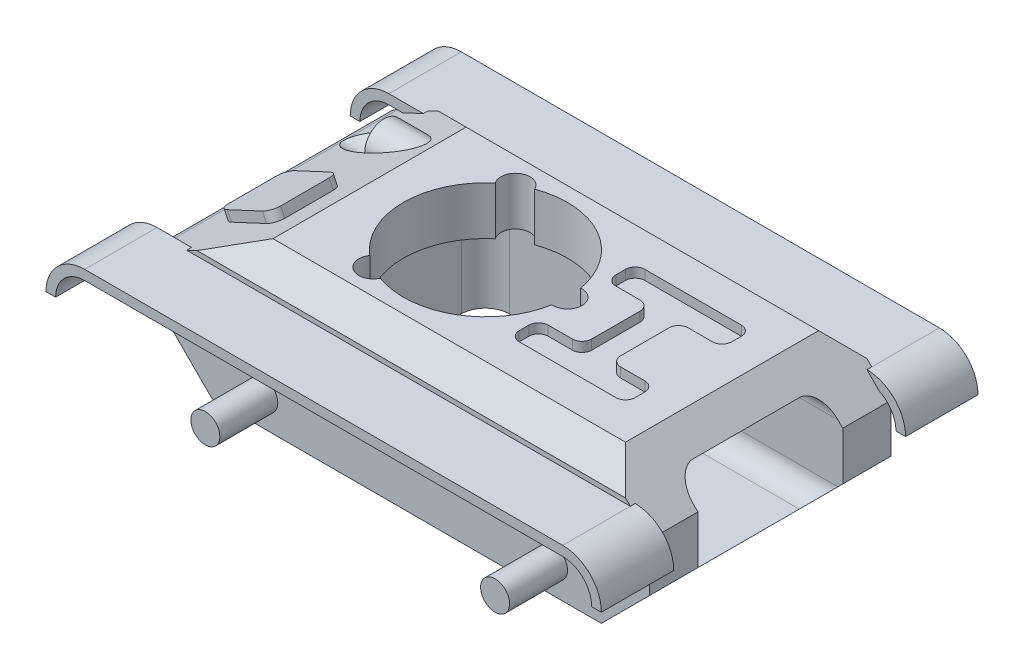
SolidWorks part; units mm, degrees
ref_plane "Front Plane" through (0, 0, 0) normal (0, 0, 1) x (1, 0, 0)
ref_plane "Top Plane" through (0, 0, 0) normal (0, 1, 0) x (1, 0, 0)
ref_plane "Right Plane" through (0, 0, 0) normal (1, 0, 0) x (0, 0, -1)
sketch "Sketch1" plane through (0, 0, 0) normal (0, 0, 1) x (1, 0, 0)
  line L0 (0, 0) -> (-80.6266, 0)
  line L1 (-80.6266, 0) -> (-93.6115, 12.9849)
  line L2 (-92.1891, 21.052) -> (-73, 30)
  line L3 (-73, 30) -> (0, 30)
  line L4 (0, 30) -> (10, 20)
  line L5 (10, 20) -> (10, 10)
  line L6 (10, 10) -> (0, 0)
  arc A0 (-92.1891, 21.052) -> (-93.6115, 12.9849) centre (-90.076, 16.5205) ccw
  point P12 (-95, 17.3887)
  dimension "D2" = 5
  dimension "D1" = 70
  dimension "D3" = 30
  dimension "D4" = 45
  dimension "D5" = 45
  dimension "D6" = 10
  dimension "D7" = 45
  dimension "D8" = 10
  dimension "D9" = 105
  dimension "D10" = 22
extrude "Boss-Extrude1" add sketch "Sketch1" along normal mid plane 50
chamfer "Chamfer1" distance 5 angle 45 2 edges at (-36.5, 30, 25) (-36.5, 30, -25)
sketch "Sketch2" plane through (0, 30, 0) normal (0, 1, 0) x (1, 0, 0)
  line L4 (-14, -7) -> (-9, -7)
  line L5 (-7, -9) -> (-7, -11)
  line L6 (-9, -13) -> (-29, -13)
  line L7 (-31, -11) -> (-31, -9)
  line L8 (-29, -7) -> (-24, -7)
  line L9 (-22, -5) -> (-22, 5)
  line L12 (10, -25) -> (10, 25) construction
  line L13 (-49, 0) -> (21.9444, 0) construction
  line L14 (-16, -5) -> (-16, 5)
  line L15 (-29, 7) -> (-24, 7)
  line L16 (-31, 11) -> (-31, 9)
  line L17 (-9, 13) -> (-29, 13)
  line L18 (-7, 9) -> (-7, 11)
  line L19 (-14, 7) -> (-9, 7)
  arc A0 (-59.9556, 12.999) -> (-59.9556, -12.999) centre (-49, 0) ccw
  arc A3 (-7, -11) -> (-9, -13) centre (-9, -11) cw
  arc A4 (-9, -7) -> (-7, -9) centre (-9, -9) cw
  arc A5 (-29, -13) -> (-31, -11) centre (-29, -11) cw
  arc A6 (-31, -9) -> (-29, -7) centre (-29, -9) cw
  arc A7 (-24, -7) -> (-22, -5) centre (-24, -5) ccw
  arc A8 (-16, -5) -> (-14, -7) centre (-14, -5) ccw
  arc A9 (-31, 9) -> (-29, 7) centre (-29, 9) ccw
  arc A10 (-29, 13) -> (-31, 11) centre (-29, 11) ccw
  arc A11 (-7, 11) -> (-9, 13) centre (-9, 11) ccw
  arc A12 (-9, 7) -> (-7, 9) centre (-9, 9) ccw
  arc A13 (-24, 7) -> (-22, 5) centre (-24, 5) cw
  arc A14 (-16, 5) -> (-14, 7) centre (-14, 5) cw
  arc A15 (-32.2647, -2.9883) -> (-32.2647, 2.9883) centre (-32, 0) ccw
  arc A16 (-59.9556, -12.999) -> (-54.7797, -15.9873) centre (-57.5, -14.7224) ccw
  arc A17 (-54.7797, 15.9873) -> (-59.9556, 12.999) centre (-57.5, 14.7224) ccw
  arc A18 (-32.2647, 2.9883) -> (-54.7797, 15.9873) centre (-49, 0) ccw
  arc A19 (-54.7797, -15.9873) -> (-32.2647, -2.9883) centre (-49, 0) ccw
  arc A20 (-59.9556, -12.999) -> (-54.7797, -15.9873) centre (-49, 0) ccw construction
  point P1 (-22, 0)
  point P11 (-7, -13)
  point P13 (-19, -13)
  point P16 (-7, -7)
  point P23 (-31, -13)
  point P30 (-16, -7)
  point P50 (-16, 0)
  point P61 (-49, 0)
  dimension "D4" = 34
  dimension "D8" = 6
  dimension "D7" = 2
  dimension "D1" = 24
  dimension "D2" = 6
  dimension "D3" = 13
  dimension "D5" = 59
  dimension "D6" = 30
  dimension "D9" = 6
  dimension "D10" = 3
sketch "Sketch3" plane through (-24.5289, 52.6024, 0) normal (-0.4226, 0.9063, 0) x (0.9063, 0.4226, 0)
  line L1 (-68.4819, -15) -> (-60.4819, -15)
  line L2 (-70.4819, -13) -> (-70.4819, -3)
  line L3 (-68.4819, -1) -> (-60.4819, -1)
  line L4 (-58.4819, -13) -> (-58.4819, -3)
  line L5 (-70.4819, -15) -> (-58.4819, -1) construction
  line L6 (-70.4819, -1) -> (-58.4819, -15) construction
  line L7 (-53.4819, -20) -> (-53.4819, 20) construction
  arc A0 (-60.4819, -15) -> (-58.4819, -13) centre (-60.4819, -13) ccw
  arc A1 (-68.4819, -15) -> (-70.4819, -13) centre (-68.4819, -13) cw
  arc A2 (-70.4819, -3) -> (-68.4819, -1) centre (-68.4819, -3) cw
  arc A3 (-60.4819, -1) -> (-58.4819, -3) centre (-60.4819, -3) cw
  point P0 (-64.4819, -8)
  dimension "D4" = 2
  dimension "D1" = 11
  dimension "D2" = 12
  dimension "D3" = 14
  dimension "D5" = 8
extrude "Boss-Extrude2" add sketch "Sketch3" along normal blind 2
extrude "Cut-Extrude1" cut sketch "Sketch2" against normal blind 2
sketch "Sketch4" plane through (0, 28, 0) normal (0, 1, 0) x (1, 0, 0)
  arc A6 (-54.7797, -15.9873) -> (-32.2647, -2.9883) centre (-49, 0) ccw
  arc A7 (-32.2647, -2.9883) -> (-32.2647, 2.9883) centre (-32, 0) ccw
  arc A8 (-32.2647, 2.9883) -> (-54.7797, 15.9873) centre (-49, 0) ccw
  arc A9 (-54.7797, 15.9873) -> (-59.9556, 12.999) centre (-57.5, 14.7224) ccw
  arc A10 (-59.9556, 12.999) -> (-59.9556, -12.999) centre (-49, 0) ccw
  arc A11 (-59.9556, -12.999) -> (-54.7797, -15.9873) centre (-57.5, -14.7224) ccw
  arc A12 (-54.7797, -15.9873) -> (-32.2647, -2.9883) centre (-49, 0) ccw
  arc A13 (-32.2647, -2.9883) -> (-32.2647, 2.9883) centre (-32, 0) ccw
  arc A14 (-32.2647, 2.9883) -> (-54.7797, 15.9873) centre (-49, 0) ccw
  arc A15 (-54.7797, 15.9873) -> (-59.9556, 12.999) centre (-57.5, 14.7224) ccw
  arc A16 (-59.9556, 12.999) -> (-59.9556, -12.999) centre (-49, 0) ccw
  arc A17 (-59.9556, -12.999) -> (-54.7797, -15.9873) centre (-57.5, -14.7224) ccw
  dimension "D1" = 0
extrude "Cut-Extrude2" cut sketch "Sketch4" against normal blind 8
sketch "Sketch5" plane through (10, 0, 0) normal (1, 0, 0) x (0, 0, -1)
  line L0 (-25, 0) -> (25, 0) construction
  line L1 (-11, 5) -> (11, 5)
  line L2 (-15, 9) -> (-15, 21)
  line L3 (-11, 25) -> (11, 25)
  line L4 (15, 9) -> (15, 21)
  line L5 (-15, 5) -> (15, 25) construction
  line L6 (-15, 25) -> (15, 5) construction
  arc A0 (-11, 5) -> (-15, 9) centre (-11, 9) cw
  arc A1 (11, 5) -> (15, 9) centre (11, 9) ccw
  arc A2 (11, 25) -> (15, 21) centre (11, 21) cw
  arc A3 (-15, 21) -> (-11, 25) centre (-11, 21) cw
  point P0 (0, 15)
  dimension "D4" = 4
  dimension "D1" = 20
  dimension "D2" = 30
  dimension "D3" = 15
extrude "Cut-Extrude3" cut sketch "Sketch5" against normal blind 38
sketch "Sketch6" plane through (0, 0, 0) normal (0, -1, 0) x (1, 0, 0)
  line L0 (10, 25) -> (10, 15) construction
  line L1 (-65, -21) -> (-33, -21)
  line L2 (-70, -16) -> (-70, 16)
  line L3 (-65, 21) -> (-33, 21)
  line L4 (-28, -16) -> (-28, 16)
  line L5 (-70, -21) -> (-28, 21) construction
  line L6 (-70, 21) -> (-28, -21) construction
  arc A0 (-65, -21) -> (-70, -16) centre (-65, -16) cw
  arc A1 (-33, -21) -> (-28, -16) centre (-33, -16) ccw
  arc A2 (-33, 21) -> (-28, 16) centre (-33, 16) cw
  arc A3 (-70, 16) -> (-65, 21) centre (-65, 16) cw
  point P0 (-49, 0)
  dimension "D4" = 5
  dimension "D1" = 59
  dimension "D2" = 42
  dimension "D3" = 42
extrude "Cut-Extrude4" cut sketch "Sketch6" against normal blind 20
sketch "Sketch7" plane through (10, 0, 0) normal (1, 0, 0) x (0, 0, -1)
  line L1 (-20, 30) -> (20, 30) construction
  circle A0 centre (14, 25) radius 4
  dimension "D1" = 8
  dimension "D2" = 14
  dimension "D3" = 5
extrude "Cut-Extrude6" cut sketch "Sketch7" against normal blind 30 from offset 80 offset against normal yes
sketch "Sketch8" plane through (0, 0, 25) normal (0, 0, 1) x (1, 0, 0)
  line L0 (-93, 24) -> (6, 24)
  line L1 (-80.6266, 0) -> (0, 0) construction
  line L2 (10, 10) -> (10, 20) construction
  line L3 (-93, 22) -> (6, 22)
  line L4 (-101, 16) -> (-99, 16)
  line L5 (12, 16) -> (14, 16)
  arc A0 (-101, 16) -> (-93, 24) centre (-93, 16) cw
  arc A1 (6, 24) -> (14, 16) centre (6, 16) cw
  arc A2 (-99, 16) -> (-93, 22) centre (-93, 16) cw
  arc A3 (6, 22) -> (12, 16) centre (6, 16) cw
  dimension "D2" = 8
  dimension "D1" = 16
  dimension "D3" = 24
  dimension "D4" = 103
  dimension "D5" = 115
  dimension "D6" = 2
extrude "Boss-Extrude3" add sketch "Sketch8" along normal blind 14 and the other way blind 1
sketch "Sketch9" plane through (0, 0, 25) normal (0, 0, 1) x (1, 0, 0)
  line L0 (-80.6266, 0) -> (0, 0) construction
  line L1 (10, 10) -> (10, 20) construction
  circle A0 centre (-70, 6) radius 3
  arc A1 (-93, 24) -> (-101, 16) centre (-93, 16) ccw construction
  circle A2 centre (-10, 6) radius 3
  dimension "D2" = 6
  dimension "D5" = 6
  dimension "D1" = 6
  dimension "D3" = 23
  dimension "D4" = 6
  dimension "D6" = 20
extrude "Boss-Extrude4" add sketch "Sketch9" along normal blind 12
mirror "Mirror1" about plane through (0, 0, 0) normal (0, 0, 1) of "Boss-Extrude3", "Boss-Extrude4"
sketch "Sketch10" plane through (-70, 0, 0) normal (-1, 0, 0) x (0, 0, 1)
  circle A0 centre (-14, 25) radius 4 construction
  circle A1 centre (-14, 25) radius 4
  circle A2 centre (-14, 25) radius 3
  dimension "D1" = 1
extrude "Boss-Extrude5" add sketch "Sketch10" along normal blind 14
